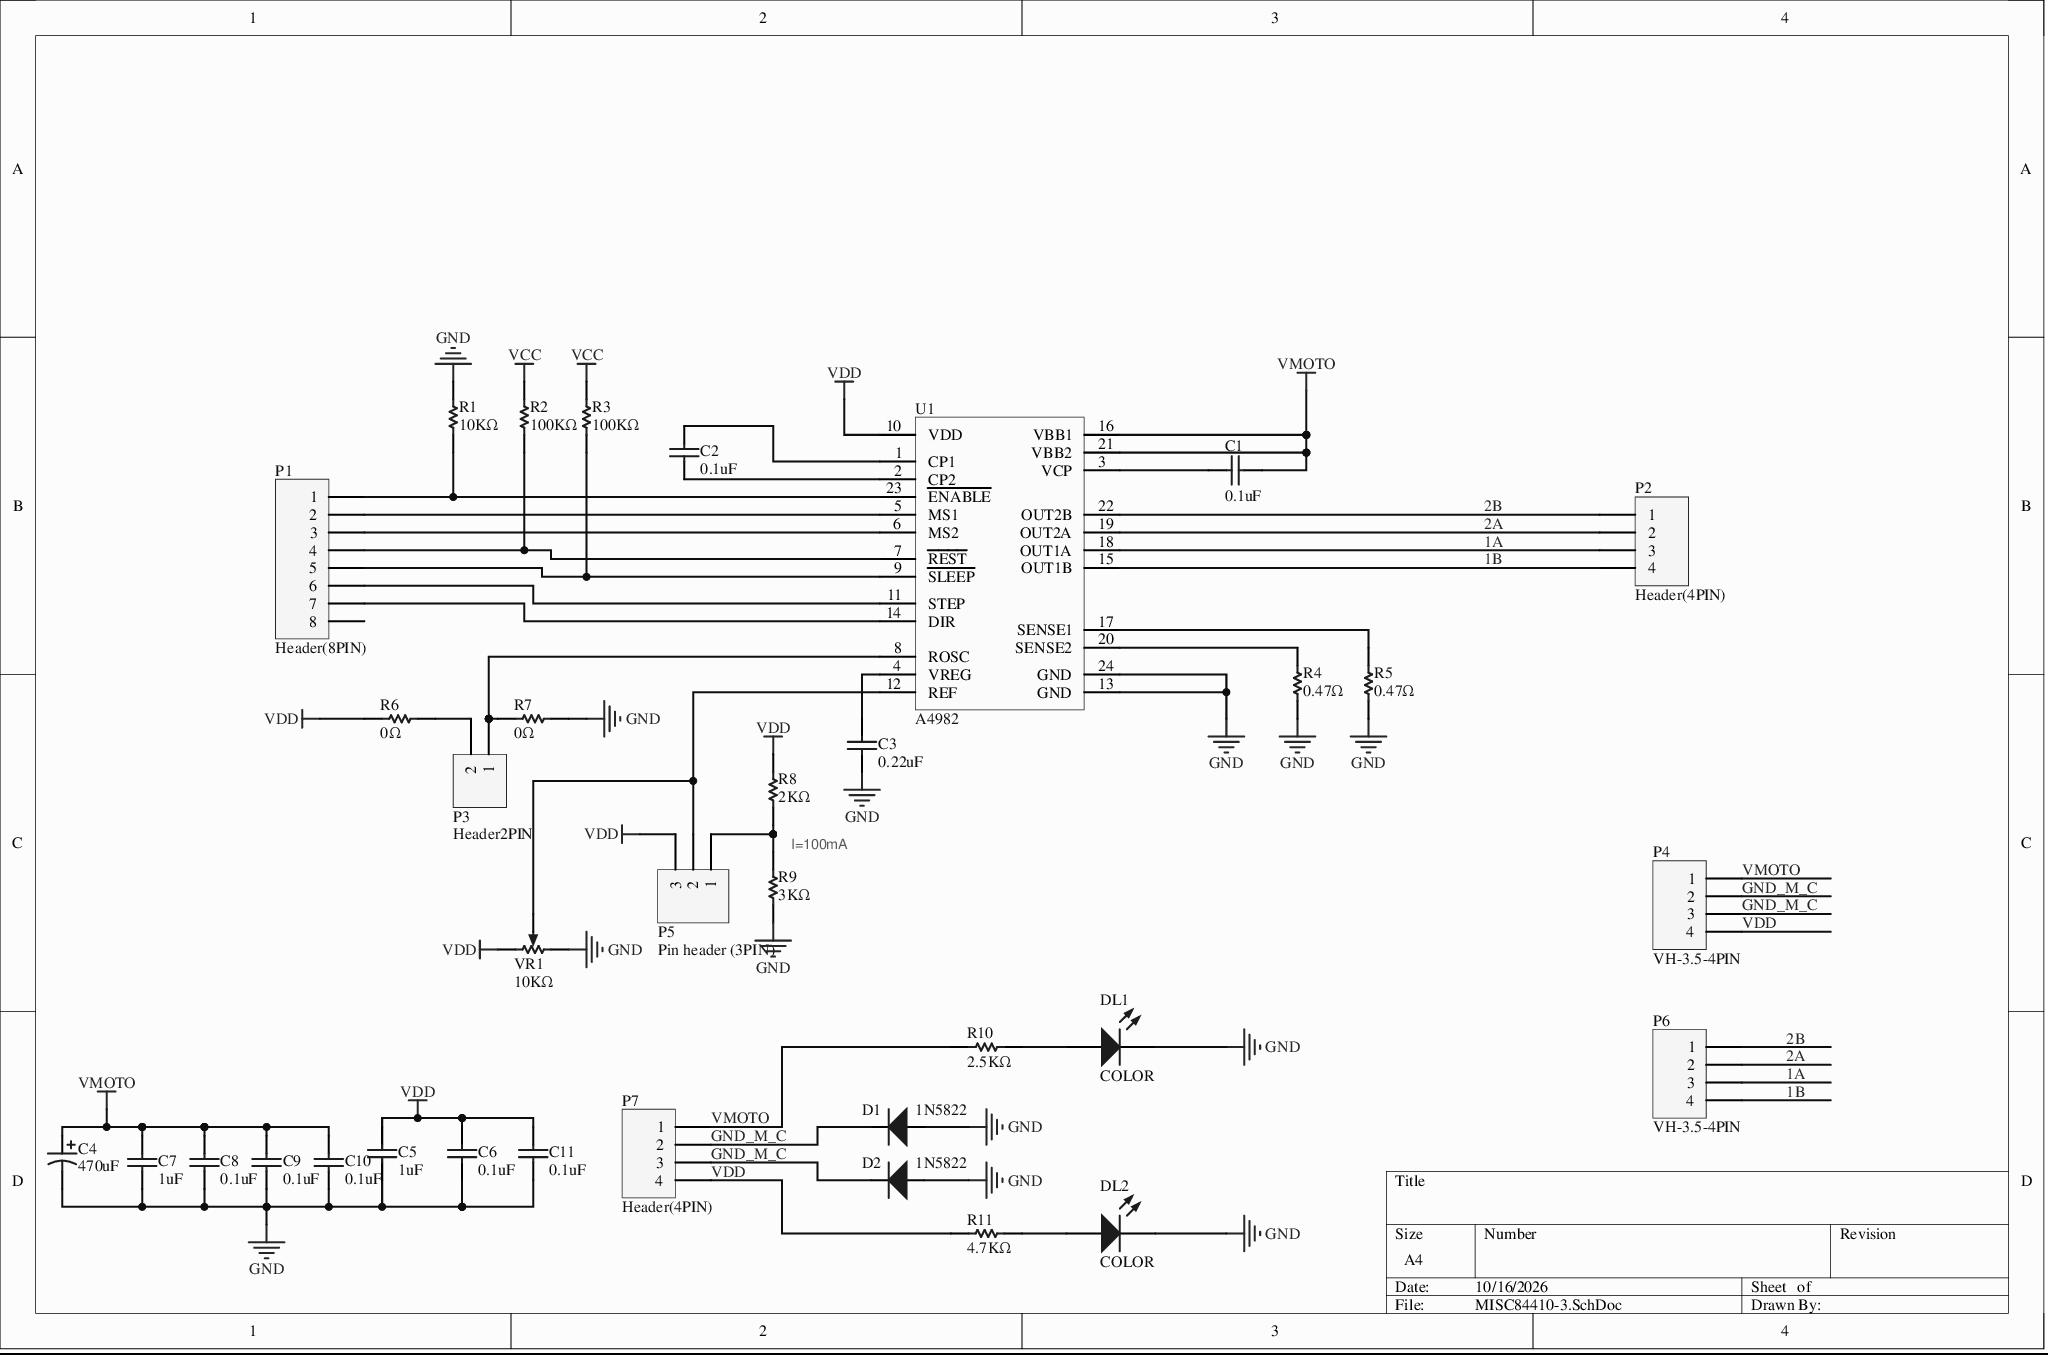
[diagram p0: MISC84410-3.SchDoc]
# Altium project MISC84410-2.PrjPcb
1 sheet, 35 parts. Net scope: global (net labels, ports and power ports of the same name join across sheets).
Board file: MISC84410.PcbDoc

## Sheet MISC84410-3.SchDoc
size A4

### Parts
C1  0.1uF  [0805C]
C2  0.1uF  [0805C]
C3  0.22uF  [0805C]
C4  470uF  [CAP-SMD Aluminum Capacitors F8 220uF 35V]
C5  1uF  [0805C]
C6  0.1uF  [0805C]
C7  1uF  [0805C]
C8  0.1uF  [0805C]
C9  0.1uF  [0805C]
C10  0.1uF  [0805C]
C11  0.1uF  [0805C]
D1  1N5822  [1N5822]
D2  1N5822  [1N5822]
DL1  COLOR  [0805D]
DL2  COLOR  [0805D]
P1  Header(8PIN)  [排针（8PIN）]
P2  Header(4PIN)  [排针(4PIN)]
P3  Header2PIN  [排针2PIN]
P4  VH-3.5-4PIN  [VH-3.5-4PIN]
P5  Pin header (3PIN)  [排针(3PIN)]
P6  VH-3.5-4PIN  [VH-3.5-4PIN]
P7  Header(4PIN)  [排针(4PIN)]
R1  10KΩ  [0805R]
R2  100KΩ  [0805R]
R3  100KΩ  [0805R]
R4  0.47Ω  [0805R]
R5  0.47Ω  [0805R]
R6  0Ω  [0805R]
R7  0Ω  [0805R]
R8  2KΩ  [0805R]
R9  3KΩ  [0805R]
R10  2.5KΩ  [0805R]
R11  4.7KΩ  [0805R]
U1  value A4982  [A4982]  (hidden comment: Value)
VR1  10KΩ  [3224W]

### Nets
GND: C3.2 C4.2 C5.2 C6.2 C7.2 C8.2 C9.2 C10.2 C11.2 D1.1(A) D2.1(A) DL1.2(K) DL2.2(K) R1.2 R4.1 R5.1 R7.1 R9.2 U1.13(GND) U1.24(GND) VR1.1(TOP)
VCC: R2.2 R3.2
VDD: C5.1 C6.1 C11.1 P4.4 P5.3 P7.4 R6.2 R8.1 R11.1 U1.10(VDD) VR1.3(BOT)
VMOTO: C1.1 C4.1 C7.1 C8.1 C9.1 C10.1 P4.1 P7.1 R10.1 U1.16(VBB1) U1.21(VBB2)
1A: P2.3 P6.3 U1.18(OUT1A)
1B: P2.4 P6.4 U1.15(OUT1B)
2A: P2.2 P6.2 U1.19(OUT2A)
2B: P2.1 P6.1 U1.22(OUT2B)
GND_M_C: D1.2(K) D2.2(K) P4.2 P4.3 P7.2 P7.3
NetC1_2: C1.2 U1.3(VCP)
NetC2_1: C2.1 U1.2(CP2)
NetC2_2: C2.2 U1.1(CP1)
NetC3_1: C3.1 U1.4(VREG)
NetDL1_1: DL1.1(A) R10.2
NetDL2_1: DL2.1(A) R11.2
NetP1_1: P1.1 R1.1 U1.23(~{ENABLE})
NetP1_2: P1.2 U1.5(MS1)
NetP1_3: P1.3 U1.6(MS2)
NetP1_4: P1.4 R2.1 U1.7(~{REST})
NetP1_5: P1.5 R3.1 U1.9(~{SLEEP})
NetP1_6: P1.6 U1.11(STEP)
NetP1_7: P1.7 U1.14(DIR)
NetP3_1: P3.1 R7.2 U1.8(ROSC)
NetP3_2: P3.2 R6.1
NetP5_1: P5.1 R8.2 R9.1
NetP5_2: P5.2 U1.12(REF) VR1.2(TAP)
NetR4_2: R4.2 U1.20(SENSE2)
NetR5_2: R5.2 U1.17(SENSE1)

Not connected (* = marked no-connect by the designer): P1 8

### Notes on the sheet
- I=100mA

### Library data of the parts
C1-C3 C5-C11 = CAP0805: 0805 SMD capacitor
  C1 C2 C6 C8-C11: Value: 0.1uF
  C3: Value: 0.22uF
  C5 C7: Value: 1uF
C4 = CAP-AEC: THT capacitor; Value: 470uF
D1 D2 = IN5822: Value: 1N5822
DL1 DL2 = LED_0805: Value: COLOR
P1 = Header 8: Header, 8-Pin; LatestRevisionDate: 17-Jul-2002; LatestRevisionNote: Re-released for DXP Platform.; Publisher: Altium Limited
P2 P4 P6 P7 = Header 4: Header, 4-Pin; LatestRevisionDate: 17-Jul-2002; LatestRevisionNote: Re-released for DXP Platform.; Publisher: Altium Limited
P3 = Header 2: Header, 2-Pin; LatestRevisionDate: 17-Jul-2002; LatestRevisionNote: Re-released for DXP Platform.; Publisher: Altium Limited
P5 = Header 3: LatestRevisionDate: 17-Jul-2002; LatestRevisionNote: Re-released for DXP Platform.; Publisher: Altium Limited
R1-R11 = RES0805: 0805 SMD resistor
  R1: Value: 10KΩ
  R2 R3: Value: 100KΩ
  R4 R5: Value: 0.47Ω
  R6 R7: Value: 0Ω
  R8: Value: 2KΩ
  R9: Value: 3KΩ
  R10: Value: 2.5KΩ
  R11: Value: 4.7KΩ
U1 = A4982
VR1 = RPOT: RPOT-SMD-10KΩ; Value: 10KΩ